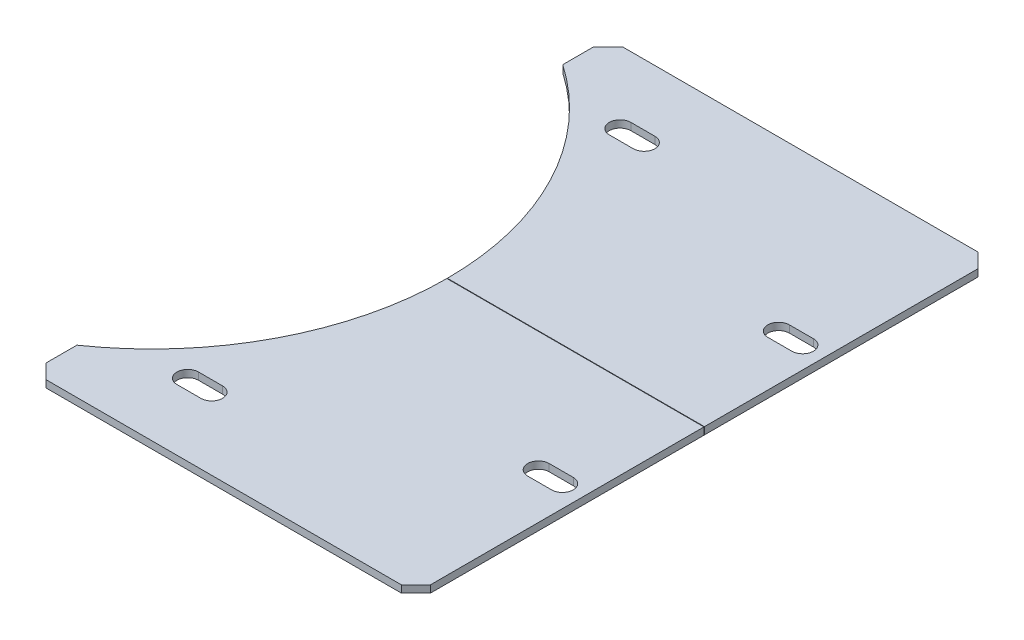
from build123d import *

# Parameters (mm, degrees)
SKETCH1_W           = 552
SKETCH1_H           = 120
BOSS_EXTRUDE1_DEPTH = 1.5
CHAMFER1_SIZE       = 3
CHAMFER2_SIZE       = 3
CUT_EXTRUDE6_DEPTH  = 283.45043813
SKETCH13_W          = 552
SKETCH13_H          = 0.1
CUT_EXTRUDE7_DEPTH  = 283.45043813
CUT_EXTRUDE9_DEPTH  = 283.45043813
SKETCH16_R          = 61.5
CUT_EXTRUDE10_DEPTH = 10
SKETCH18_W          = 998.789859015
SKETCH18_H          = 252.863725976
CUT_EXTRUDE11_DEPTH = 10
CUT_EXTRUDE12_DEPTH = 10
CHAMFER3_SIZE       = 3
CHAMFER4_SIZE       = 3


with BuildPart() as part:
    # Sketch1 → Boss-Extrude1 (new body)
    with BuildSketch(Plane(origin=(0, 0, 0), x_dir=(1, 0, 0), z_dir=(0, 1, 0))):
        Rectangle(SKETCH1_W, SKETCH1_H)
    extrude(amount=BOSS_EXTRUDE1_DEPTH)

    # Chamfer1
    chamfer1_edges = [part.edges().sort_by_distance(p)[0] for p in [
        (276, 0.75, 60),
        (276, 0.75, -60),
    ]]
    chamfer(chamfer1_edges, length=CHAMFER1_SIZE)

    # Chamfer2
    chamfer2_edges = [part.edges().sort_by_distance(p)[0] for p in [
        (-276, 0.75, 60),
        (-276, 0.75, -60),
    ]]
    chamfer(chamfer2_edges, length=CHAMFER2_SIZE)

    # Sketch12 → Cut-Extrude6 (cut, through all)
    with BuildSketch(Plane(origin=(0, 1.5, 0), x_dir=(1, 0, 0), z_dir=(0, 1, 0))):
        with BuildLine():
            Line((-258.5, 47.25), (-253.5, 47.25))
            ThreePointArc((-253.5, 47.25), (-251.25, 45), (-253.5, 42.75))
            Line((-253.5, 42.75), (-258.5, 42.75))
            ThreePointArc((-258.5, 42.75), (-260.75, 45), (-258.5, 47.25))
        make_face()
        with BuildLine():
            Line((-258.5, -42.75), (-253.5, -42.75))
            ThreePointArc((-253.5, -42.75), (-251.25, -45), (-253.5, -47.25))
            Line((-253.5, -47.25), (-258.5, -47.25))
            ThreePointArc((-258.5, -47.25), (-260.75, -45), (-258.5, -42.75))
        make_face()
    extrude(amount=-CUT_EXTRUDE6_DEPTH, mode=Mode.SUBTRACT)

    # Sketch13 → Cut-Extrude7 (cut, through all)
    with BuildSketch(Plane(origin=(0, 1.5, 0), x_dir=(1, 0, 0), z_dir=(0, 1, 0))):
        Rectangle(SKETCH13_W, SKETCH13_H)
    extrude(amount=-CUT_EXTRUDE7_DEPTH, mode=Mode.SUBTRACT)


with BuildPart() as cut_extrude7_piece_1:
    # of the separate pieces the step leaves, piece 1, a body of its own (cut_extrude7_pieces)
    add(part.part.solids().sort_by_distance((-273, 0, -60))[0])


with BuildPart() as cut_extrude7_piece_2:
    # of the separate pieces the step leaves, piece 2, a body of its own (cut_extrude7_pieces)
    add(part.part.solids().sort_by_distance((-276, 0, 57))[0])


with BuildPart() as cut_extrude9_tool:
    # Sketch15 → Cut-Extrude9 (new, through all)
    with BuildSketch(Plane(origin=(0, 1.5, 0), x_dir=(1, 0, 0), z_dir=(0, 1, 0))):
        with BuildLine():
            Line((52, 35.95), (-14, 35.95))
            ThreePointArc((-14, 35.95), (-16.121320344, 35.071320344), (-17, 32.95))
            Line((-17, 32.95), (-17, -33.05))
            ThreePointArc((-17, -33.05), (-16.121320344, -35.171320344), (-14, -36.05))
            Line((-14, -36.05), (52, -36.05))
            ThreePointArc((52, -36.05), (54.121320344, -35.171320344), (55, -33.05))
            Line((55, -33.05), (55, 32.95))
            ThreePointArc((55, 32.95), (54.121320344, 35.071320344), (52, 35.95))
        make_face()
    extrude(amount=-CUT_EXTRUDE9_DEPTH)


with BuildPart() as cut_extrude7_piece_1_1:
    add(cut_extrude7_piece_1.part)

    # Cut-Extrude9: cut by cut_extrude9_tool
    add(cut_extrude9_tool.part, mode=Mode.SUBTRACT)


with BuildPart() as cut_extrude7_piece_2_1:
    add(cut_extrude7_piece_2.part)

    # Cut-Extrude9: cut by cut_extrude9_tool
    add(cut_extrude9_tool.part, mode=Mode.SUBTRACT)


with BuildPart() as cut_extrude10_tool:
    # Sketch16 → Cut-Extrude10 (new body)
    with BuildSketch(Plane(origin=(0, 1.5, 0), x_dir=(1, 0, 0), z_dir=(0, 1, 0))):
        with Locations((311, 0)):
            Circle(SKETCH16_R)
        with Locations((-311, 0)):
            Circle(SKETCH16_R)
    extrude(amount=-CUT_EXTRUDE10_DEPTH)


with BuildPart() as cut_extrude7_piece_1_2:
    add(cut_extrude7_piece_1_1.part)

    # Cut-Extrude10: cut by cut_extrude10_tool
    add(cut_extrude10_tool.part, mode=Mode.SUBTRACT)


with BuildPart() as cut_extrude7_piece_2_2:
    add(cut_extrude7_piece_2_1.part)

    # Cut-Extrude10: cut by cut_extrude10_tool
    add(cut_extrude10_tool.part, mode=Mode.SUBTRACT)


with BuildPart() as cut_extrude11_tool:
    # Sketch18 → Cut-Extrude11 (new body)
    with BuildSketch(Plane.XZ):
        with Locations((303.394929508, 0)):
            Rectangle(SKETCH18_W, SKETCH18_H)
    extrude(amount=-CUT_EXTRUDE11_DEPTH)


with BuildPart() as cut_extrude7_piece_1_3:
    add(cut_extrude7_piece_1_2.part)

    # Cut-Extrude11: cut by cut_extrude11_tool
    add(cut_extrude11_tool.part, mode=Mode.SUBTRACT)


with BuildPart() as cut_extrude7_piece_2_3:
    add(cut_extrude7_piece_2_2.part)

    # Cut-Extrude11: cut by cut_extrude11_tool
    add(cut_extrude11_tool.part, mode=Mode.SUBTRACT)


with BuildPart() as cut_extrude12_tool:
    # Sketch17 → Cut-Extrude12 (new body)
    with BuildSketch(Plane.XZ):
        with BuildLine():
            Line((-200.5, -27.25), (-205.5, -27.25))
            ThreePointArc((-205.5, -27.25), (-207.75, -25), (-205.5, -22.75))
            Line((-205.5, -22.75), (-200.5, -22.75))
            ThreePointArc((-200.5, -22.75), (-198.25, -25), (-200.5, -27.25))
        make_face()
        with BuildLine():
            Line((-200.5, 22.75), (-205.5, 22.75))
            ThreePointArc((-205.5, 22.75), (-207.75, 25), (-205.5, 27.25))
            Line((-205.5, 27.25), (-200.5, 27.25))
            ThreePointArc((-200.5, 27.25), (-198.25, 25), (-200.5, 22.75))
        make_face()
    extrude(amount=-CUT_EXTRUDE12_DEPTH)


with BuildPart() as cut_extrude7_piece_1_4:
    add(cut_extrude7_piece_1_3.part)

    # Cut-Extrude12: cut by cut_extrude12_tool
    add(cut_extrude12_tool.part, mode=Mode.SUBTRACT)

    # Chamfer4
    chamfer4_edges = [cut_extrude7_piece_1_4.edges().sort_by_distance(p)[0] for p in [
        (-196, 0.75, -60),
    ]]
    chamfer(chamfer4_edges, length=CHAMFER4_SIZE)


with BuildPart() as cut_extrude7_piece_2_4:
    add(cut_extrude7_piece_2_3.part)

    # Cut-Extrude12: cut by cut_extrude12_tool
    add(cut_extrude12_tool.part, mode=Mode.SUBTRACT)

    # Chamfer3
    chamfer3_edges = [cut_extrude7_piece_2_4.edges().sort_by_distance(p)[0] for p in [
        (-196, 0.75, 60),
    ]]
    chamfer(chamfer3_edges, length=CHAMFER3_SIZE)


solid = Compound([cut_extrude7_piece_1_4.part, cut_extrude7_piece_2_4.part])
